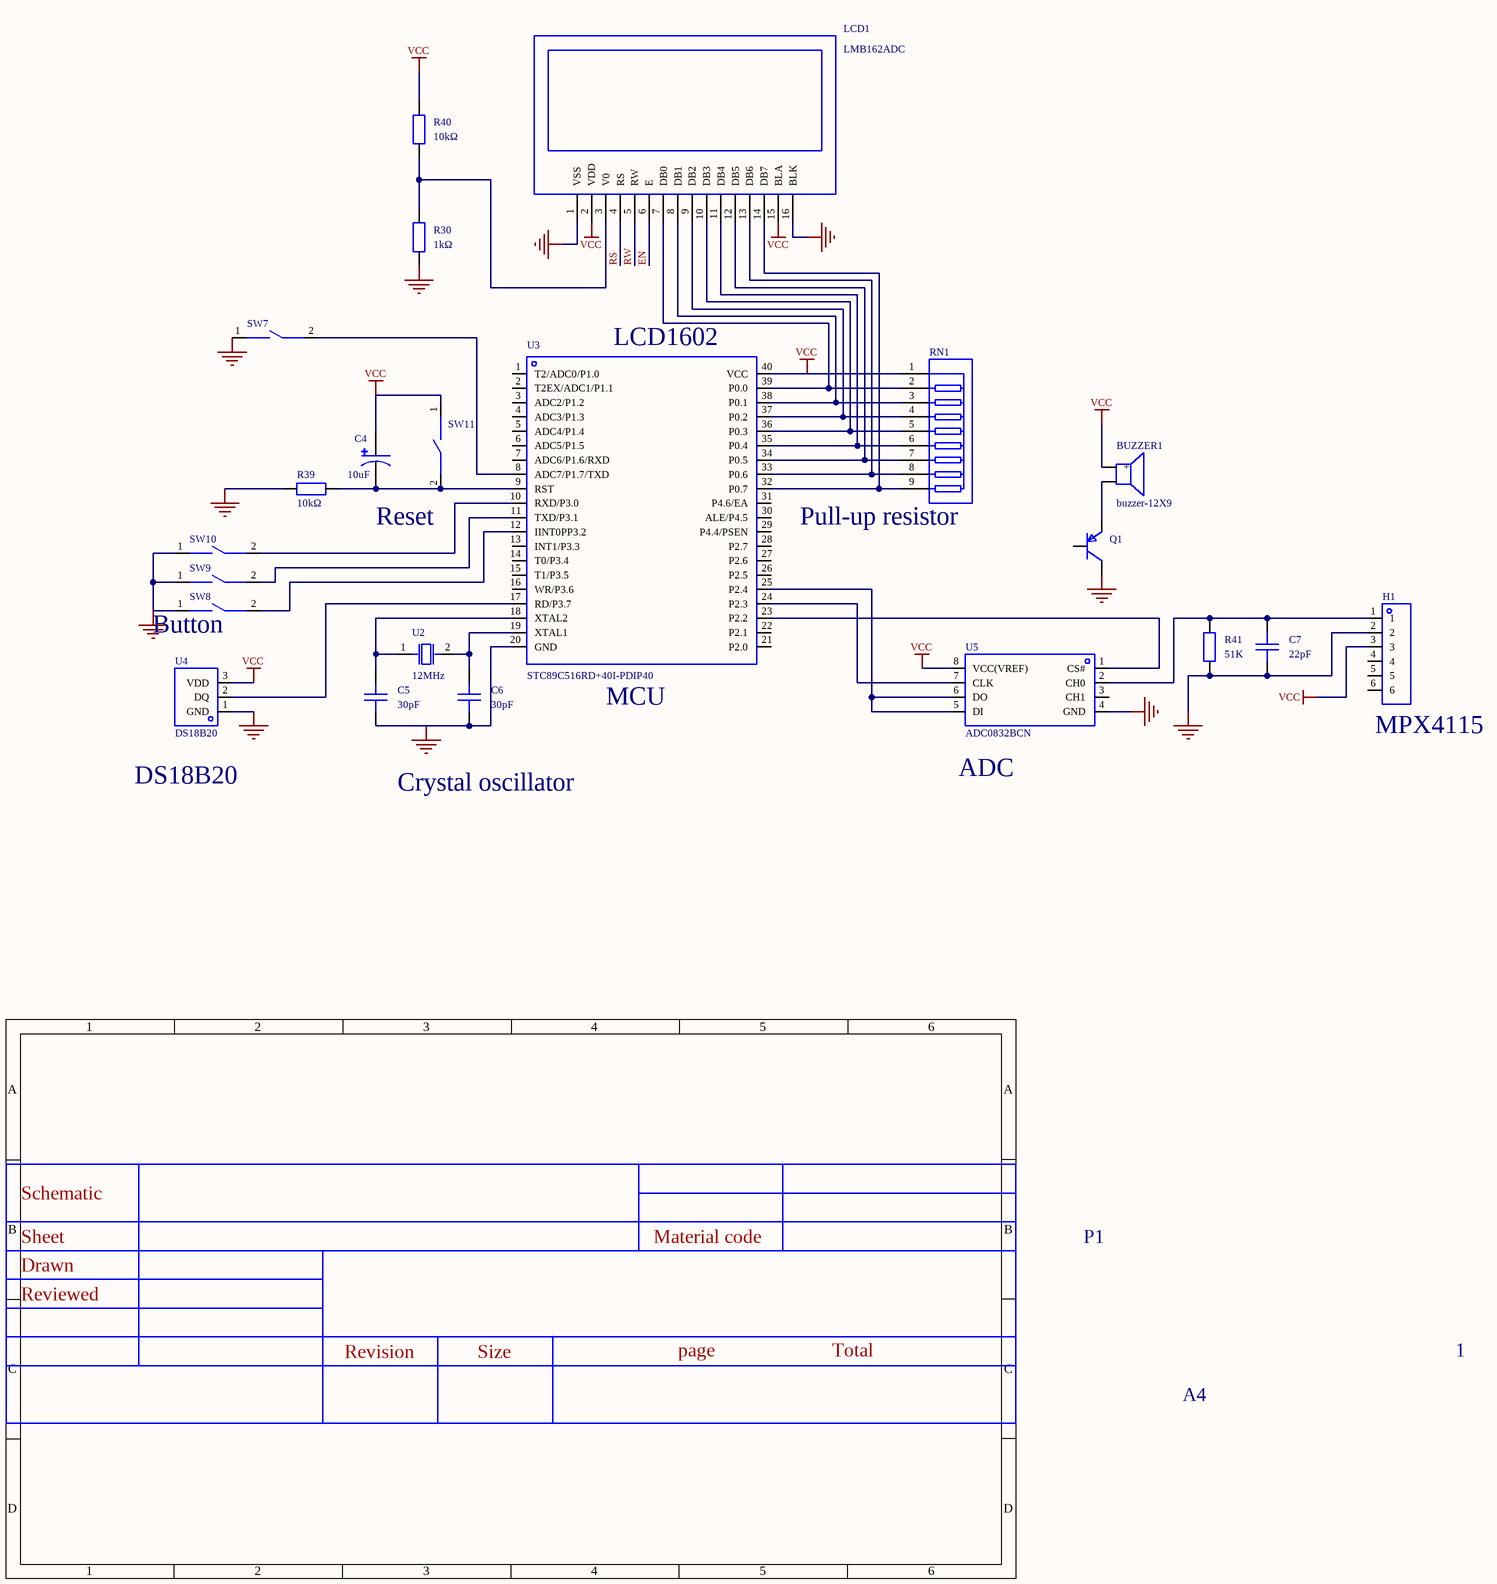
[diagram p0: MISC49895-3.schdoc]
# Altium project MISC49895-2.PrjPcb
1 sheet, 22 parts. Net scope: global (net labels, ports and power ports of the same name join across sheets).
Board file: MISC49895.pcbdoc

## Sheet MISC49895-3.schdoc
size 178 x 98 mm; Version: V1.0; @Project Name: MISC49895; @Page Count: 1; @Update Date: 2025-06-22; @Create Date: 2025-06-22; @Schematic Name: MISC49895; @Page No: 1; @Board Name: MISC49895; @Create Time: 22:14:13; @Update Time: 18:45:29

### Parts
BUZZER1  buzzer-12X9  [BUZ-TH_BD12.0-P7.60-D0.6-FD]
C4  10uF  [CAP-TH_BD6.3-P2.50-D1.0-FD]
C5  30pF  [CAP-TH_L3.6-W2.3-P5.00-D0.5]
C6  30pF  [CAP-TH_L3.6-W2.3-P5.00-D0.5]
C7  22pF  [C0603]
H1  (no value)  [HDR-TH_6P-P2.54-V-F]
LCD1  LMB162ADC  [LCD1602]
Q1  (no value)  [S8550P_SOT]
R30  1kΩ  [Res_1/8W]
R39  10kΩ  [Res_1/8W]
R40  10kΩ  [Res_1/8W]
R41  51K  [R0603]
RN1  -  [RES-ARRAY-TH_9P-P2.54-D1.0]
SW7  Tact switch, 6*6*5 plastic head, 260G, travel 0.25mm, through-hole, middle 2 pins  [KEY-TH_2P-L6.0-W6.0-P5.00]  (value not drawn)
SW8  Tact switch, 6*6*5 plastic head, 260G, travel 0.25mm, through-hole, middle 2 pins  [KEY-TH_2P-L6.0-W6.0-P5.00]  (value not drawn)
SW9  Tact switch, 6*6*5 plastic head, 260G, travel 0.25mm, through-hole, middle 2 pins  [KEY-TH_2P-L6.0-W6.0-P5.00]  (value not drawn)
SW10  Tact switch, 6*6*5 plastic head, 260G, travel 0.25mm, through-hole, middle 2 pins  [KEY-TH_2P-L6.0-W6.0-P5.00]  (value not drawn)
SW11  Tact switch, 6*6*5 plastic head, 260G, travel 0.25mm, through-hole, middle 2 pins  [KEY-TH_2P-L6.0-W6.0-P5.00]  (value not drawn)
U2  12MHz  [HC-49US_L11.0-W4.6-P4.88]
U3  STC89C516RD+40I-PDIP40  [DIP-40_L52.3-W13.9-P2.54-LS15.2-BL]
U4  DS18B20  [TO-92-3_L4.6-W3.6-P1.27-L-1]
U5  ADC0832BCN  [PDIP-8_L9.6-W6.4-P2.54-LS7.6-BL]

### Nets
GND: C5.1 C6.1 C7.1 H1.2 LCD1.1(VSS) LCD1.16(BLK) Q1.3(C) R30.1 R39.1 R41.1 SW7.1 SW8.1 SW9.1 SW10.1 U3.20(GND) U4.1(GND) U5.4(GND)
VCC: BUZZER1.1(+) C4.1 H1.3 LCD1.2(VDD) LCD1.15(BLA) R40.2 RN1.1 SW11.1 U3.40(VCC) U4.3(VDD) U5.8(VCC(VREF))
EN: LCD1.6(E)
RS: LCD1.4(RS)
RW: LCD1.5(RW)
NetBUZZER1_2: BUZZER1.2 Q1.2(E)
NetC4_2: C4.2 R39.2 SW11.2 U3.9(RST)
NetC5_2: C5.2 U2.1(OSC1) U3.18(XTAL2)
NetC6_2: C6.2 U2.2(OSC2) U3.19(XTAL1)
NetC7_2: C7.2 H1.1 R41.2 U5.2(CH0)
NetLCD1_3: LCD1.3(V0) R30.2 R40.1
NetLCD1_7: LCD1.7(DB0) RN1.2 U3.39(P0.0)
NetLCD1_8: LCD1.8(DB1) RN1.3 U3.38(P0.1)
NetLCD1_9: LCD1.9(DB2) RN1.4 U3.37(P0.2)
NetLCD1_10: LCD1.10(DB3) RN1.5 U3.36(P0.3)
NetLCD1_11: LCD1.11(DB4) RN1.6 U3.35(P0.4)
NetLCD1_12: LCD1.12(DB5) RN1.7 U3.34(P0.5)
NetLCD1_13: LCD1.13(DB6) RN1.8 U3.33(P0.6)
NetLCD1_14: LCD1.14(DB7) RN1.9 U3.32(P0.7)
NetSW7_2: SW7.2 U3.8(ADC7/P1.7/TXD)
NetSW8_2: SW8.2 U3.12(IINT0PP3.2)
NetSW9_2: SW9.2 U3.11(TXD/P3.1)
NetSW10_2: SW10.2 U3.10(RXD/P3.0)
NetU3_17: U3.17(RD/P3.7) U4.2(DQ)
NetU3_23: U3.23(P2.2) U5.1(CS#)
NetU3_24: U3.24(P2.3) U5.7(CLK)
NetU3_25: U3.25(P2.4) U5.5(DI) U5.6(DO)

Not connected (* = marked no-connect by the designer): H1 4 5 6; Q1 1(B); U3 1(T2/ADC0/P1.0) 2(T2EX/ADC1/P1.1) 3(ADC2/P1.2) 4(ADC3/P1.3) 5(ADC4/P1.4) 6(ADC5/P1.5) 7(ADC6/P1.6/RXD) 13(INT1/P3.3) 14(T0/P3.4) 15(T1/P3.5) 16(WR/P3.6) 21(P2.0) 22(P2.1) 26(P2.5) 27(P2.6) 28(P2.7) 29(P4.4/PSEN) 30(ALE/P4.5) 31(P4.6/EA); U5 3(CH1)

### Notes on the sheet
- (near U3) LCD1602
- Reset
- (near RN1) Pull-up resistor
- (near SW8) Button
- (near U3) MCU
- (near H1) MPX4115
- (near U4) DS18B20
- Crystal oscillator
- (near U5) ADC
- 2025-06-22
- Schematic
- Sheet
- Material code
- P1
- Reviewed
- Drawn
- Revision
- Size
- page
- Total
- A4
- 1

### Library data of the parts
BUZZER1 = buzzer-12X9: AddInBom: yes; ModelId: 16ab50e14c5b4f2c986c135bdba60e37; ModelName: BUZ-TH_D12.0-H9.5-P7.60; ModelTransform: 472.44,472.176,0,90,0,0,-0.787,0,-177.165; Symbol: BUZZER-12X9; Device: buzzer-12X9; LCSC Part Name: buzzer-12X9; SupplierPart: C9900016920; ManufacturerPart: buzzer-12X9; Supplier Footprint: BUZZER_SMT_9650B; JLCPCB Part Class: Extended library; Supplier: LCSC; ConvertToPcb: yes; FootprintName: BUZ-TH_BD12.0-P7.60-D0.6-FD
C4 = LKMC1202E100MF: Capacitance: 10uF; Tolerance: ±20%; Rated voltage: 250V; Ripple current: -; Equivalent series resistance: -;; Manufacturer: Ymin(永铭); AddInBom: yes; ModelId: 0a4db4bf24b443b3be4905be97ff10c5; ModelTransform: 248.4247,247.99777,0,0,0,0,0,0,-137.795; φD: 6.3mm; L: 12mm; Lifetime @ Temp: 9000hrs@105℃; Symbol: LKMC1202E100MF; Device: LKMC1202E100MF; LCSC Part Name: 10uF ±20% 250V; SupplierPart: C443243; ManufacturerPart: LKMC1202E100MF; Supplier Footprint: 插件,D6.3xL12mm; JLCPCB Part Class: Extended library; Datasheet: https://atta.szlcsc.com/upload/public/pdf/source/20200220/C487520_443A40905984A455D375EE990FEAA9E8.pdf; Supplier: LCSC; ConvertToPcb: yes; FootprintName: CAP-TH_BD6.3-P2.50-D1.0-FD; ModelName: CAP-TH_BD6.3-P2.50-D1.0-FD; Value: 10uF; Rated Voltage: 250V; Ripple Current: -; Equivalent Series Resistance(ESR): -; Lead Spacing: 2.5mm
C5 C6 = K300J10C0GF5UH5: Capacitance: 30pF; Tolerance: ±5%; Rated voltage: 50V; Temperature coefficient: C0G;; Manufacturer: VISHAY(威世); AddInBom: yes; ModelId: 8586b865f3f94c6bbd5d7f2c3c951380; ModelName: CAP-TH-2P-L3.6-W2.3-H6.2-P5.0; ModelTransform: 220.472,90.551,0,0,0,0,-0.005,0,-137.795; Symbol: K300J10C0GF5UH5; Device: K300J10C0GF5UH5; LCSC Part Name: 30pF ±5% 50V; SupplierPart: C1623919; ManufacturerPart: K300J10C0GF5UH5; Supplier Footprint: 插件; JLCPCB Part Class: Extended library; Datasheet: https://atta.szlcsc.com/upload/public/pdf/source/20210702/6531D680143ED60327F22057485455BA.pdf; Supplier: LCSC; ConvertToPcb: yes; FootprintName: CAP-TH_L3.6-W2.3-P5.00-D0.5; Value: 30pF; Voltage Rated: 50V; Temperature Coefficient: C0G
C7 = CAP_0603: ConvertToPcb: yes; SymbolName: CapAcitance; ModelId: ac125912035d415993ca9572d50418b1; ModelName: C0603_L1.6-W0.8-H0.8; ModelTransform: 62.992,31.496,0,0,0,0,0,0,0; Value: 22pF; Device: CAP_0603; AddInBom: yes; Supplier Footprint: 0603; FootprintName: C0603
H1 = HDR-F_2.54_1x6P: Symbol: Header-Female-2.54_1x6; ConvertToPcb: yes; ModelId: 0f5bcf94dcda47d085f24cdca1696fe9; ModelTransform: 619.684,94.488,0,0,0,0,0,0,-125.984; Device: HDR-F_2.54_1x6P; AddInBom: yes; SupplierPart: C40877; Supplier Footprint: 插件; FootprintName: HDR-TH_6P-P2.54-V-F; ModelName: HDR-TH_6P-P2.54-V-F
LCD1 = LMB162ADC: 16x2 character LCD module; AddInBom: yes; ModelId: f9d832f46a914cadb50fc4d4cefd2517; ModelTransform: 3149.6,1417.32,0,0,0,0,0,0,-118.11; Symbol: LMB162ADC; Device: LMB162ADC; LCSC Part Name: LMB162ADC; SupplierPart: C9741; ManufacturerPart: LMB162ADC; Supplier Footprint: SIP; JLCPCB Part Class: Extended library; Supplier: LCSC; ConvertToPcb: yes; FootprintName: LCD1602; ModelName: LCD1602
Q1 = S8550_SOT_PNP: Symbol: PNP; ConvertToPcb: yes; ModelId: 9c0df02d6f3e44e889da37f3e5bf5496; ModelName: SOT-23-3_L2.9-W1.4-P1.90-LS2.5-BR; ModelTransform: 98.43,114.17,37.91,0,0,0,0,0,0; Device: S8550_SOT_PNP; AddInBom: yes; Supplier Footprint: SOT-23; FootprintName: S8550P_SOT
R30 R39 R40 = Res_AXIAL-1/8W: Symbol: Resistor; ConvertToPcb: yes; ModelId: b2b5ae7ae4c642178fe0039925c86a3f; ModelName: RES-TH_BD1.8-L3.2-P7.20-D0.4; ModelTransform: 282.86,66.88,253.09,0,0,0,0,0,-191; Device: Res_AXIAL-1/8W; AddInBom: yes; Supplier Footprint: 轴向引线; FootprintName: Res_1/8W
  R30: Value: 1kΩ
  R39 R40: Value: 10kΩ
R41 = Res_0603: Symbol: Resistor; ConvertToPcb: yes; ModelId: fc143cca1e79419f9cd78b61e9279f08; ModelTransform: 31.8897,63.7794,0,90,0,0,0,0,0; Value: 51K; Device: Res_0603; AddInBom: yes; Supplier Footprint: 0603; FootprintName: R0603; ModelName: R0603
RN1 = 排阻 10 K 5%: Number of resistors: -; Resistance: -; Power per element: -;; Symbol: 10 K 5%; Device: Resistor network 10 K 5%; AddInBom: yes; ModelId: d106c67f29e14d8080ba548247a719a1; ModelName: SIP-9_L22.8-W3.0-H8.5-P2.54; ModelTransform: 917.49722,118.11,0,0,0,0,0,0,-137.795; LCSC Part Name: 10KΩ (103) ±5%; SupplierPart: C26615; ManufacturerPart: 排阻 10 K 5%; Supplier Footprint: 插件; JLCPCB Part Class: Extended library; Supplier: LCSC; ConvertToPcb: yes; FootprintName: RES-ARRAY-TH_9P-P2.54-D1.0; Number of Resistors: -; Value: -; Power(Watts): -; Number of Pins: -
SW7-SW11 = 轻触开关,6*6*5塑头,260G,行程0.25mm,直插中2脚: Symbol: SWITCH,6*6*5PLASTIC HEAD,260G, 0.25MM,DIP2; AddInBom: yes; ModelId: d13ad252cbf84dc495704a853cd2bab6; ModelName: KEY-TH_2P-L6.0-W6.0-H5.0-P5.00; ModelTransform: 236.22,236.22,0,0,0,0,0,0,-137.795; Device: Tact switch, 6*6*5 plastic head, 260G, travel 0.25mm, through-hole, middle 2 pins; LCSC Part Name: 轻触开关,6*6*5塑头,260G,行程0.25mm,直插中2脚; SupplierPart: C71845; ManufacturerPart: 轻触开关,6*6*5塑头,260G,行程0.25mm,直插中2脚; Supplier Footprint: 插件; JLCPCB Part Class: Extended library; Supplier: LCSC; ConvertToPcb: yes; FootprintName: KEY-TH_2P-L6.0-W6.0-P5.00
U2 = ECS-120-S-4: Frequency: 12MHz; Frequency tolerance (room temp): ±30ppm; External load capacitance: -; Frequency stability (full temp): ±50ppm;; Manufacturer: ECS; AddInBom: yes; ModelId: 59d05c800eee432cb051aa4925461fda; ModelName: HC-49US_L11.0-W4.7-H3.5-P4.88; ModelTransform: 432.44473,183.0705,0,0,0,0,0,0,-137.795; Equivalent Series Resistance (ESR): 60Ω; Symbol: ECS-120-S-4; Device: ECS-120-S-4; LCSC Part Name: 12MHz ±30ppm; ManufacturerPart: ECS-120-S-4; Supplier Footprint: HC-49S; JLCPCB Part Class: Extended library; Datasheet: https://atta.szlcsc.com/upload/public/pdf/source/20210402/81F084B668D60DFAE850A61100CCABAF.pdf; Supplier: LCSC; ConvertToPcb: yes; FootprintName: HC-49US_L11.0-W4.6-P4.88; Value: 12MHz; Normal temperature Frequency Tolerance: ±30ppm; External load capacitor: -; Frequency Stability(Full temperature range): ±50ppm; Operating Temperature: -10℃~+70℃
U3 = STC89C516RD+40I-PDIP40: CPU core: 51 series; Program memory capacity: 61KB; Total RAM: 1.25KB; GPIO port count: 35; Operating voltage range: 3.5V~5.5V; Max CPU clock: -; Program memory type: FLASH;; Manufacturer: STC(宏晶); AddInBom: yes; ModelId: 16d4686a009b4ddca948f91eddb57b14; ModelName: DIP-40_L52.3-W13.8-H4.0-LS15.24-P2.54; ModelTransform: 2059.051,615.743,0,0,0,0,0,0,-129.921; GPIO Ports Number: 35; 16Bit Timer: 3; UART/USART: 1; Peripheral/Function: Watchdog; Symbol: STC89C516RD+40I-PDIP40; Device: STC89C516RD+40I-PDIP40; LCSC Part Name: STC89C516RD+40I-PDIP40; SupplierPart: C52225; ManufacturerPart: STC89C516RD+40I-PDIP40; Supplier Footprint: DIP-40; JLCPCB Part Class: Extended library; Datasheet: https://atta.szlcsc.com/upload/public/pdf/source/20180614/C87831_BBAF7FB8B286C29ACE4E9B180C033FEC.pdf; Supplier: LCSC; ConvertToPcb: yes; FootprintName: DIP-40_L52.3-W13.9-P2.54-LS15.2-BL; CPU Core: 51 series; Program Storage Size: 61KB; RAM Size: 1.25KB; Operating Voltage Range: 3.5V~5.5V; CPU Maximum Speed: -; Program Memory Type: FLASH; Operating Temperature Range: -40℃~+85℃; ADC (Bit): -; DAC (Bit): -; PWM (Bit): -; 8Bit Timer: -; 32Bit Timer: -; CAN: -; I2C: -; I2S: -; SPI: -; Universal Serial Bus: -; Internal Comparator: -; communication protocol: -; Watchdog: Yes; Real-Time Clock: -; Infrared Data Association: -; Low-Voltage Detect: -; CCP Capture/Compare: -; Secure Digital Input and Output: -; Direct Memory Access: -; Internal Oscillator: -
U4 = DS18B20: Temperature range: -55℃~+125℃; Accuracy: ±0.5℃; Interface type: Single-bus;; Manufacturer: Mysentech(敏源传感); Symbol: DS18B20_C20611523; AddInBom: yes; ModelId: e9e72bf1ebb8497b9f5bc8a14b0efe66; ModelTransform: 181.102,139.764,0,180,0,0,0,13.779,-196.85; Voltage - Supply: 1.8V~5.5V; Standby Current: 200nA; Device: DS18B20; LCSC Part Name: 数字温度传感芯片; SupplierPart: C20611523; ManufacturerPart: DS18B20; Supplier Footprint: TO-92; JLCPCB Part Class: Extended library; Datasheet: https://atta.szlcsc.com/upload/public/pdf/source/20240923/8CFFA5DC8B967A6FD95E1DB1474E088C.pdf; Supplier: LCSC; ConvertToPcb: yes; FootprintName: TO-92-3_L4.6-W3.6-P1.27-L-1; ModelName: TO-92-3_L4.6-W3.6-P1.27-L-1; Temperature Range: -55℃~+125℃; Tolerance: ±0.5℃; Interface: Single-bus
U5 = ADC0832BCN: Manufacturer: TI(德州仪器); AddInBom: yes; ModelId: 5dc2af053da0476fab11ee64b9a10a94; ModelName: PDIP-8_L9.6-W6.4-P2.54-LS7.62-BL; ModelTransform: 377.952,309.842,0,0,0,0,0,0,-137.795; Symbol: ADC0832BCN; Device: ADC0832BCN; LCSC Part Name: ADC0832BCN; SupplierPart: C17246630; ManufacturerPart: ADC0832BCN; Supplier Footprint: MDIP-8; Datasheet: https://atta.szlcsc.com/upload/public/pdf/source/20230922/2C7B6B6922D497DF671B03BDE4F2F9A0.pdf; Supplier: LCSC; ConvertToPcb: yes; FootprintName: PDIP-8_L9.6-W6.4-P2.54-LS7.6-BL